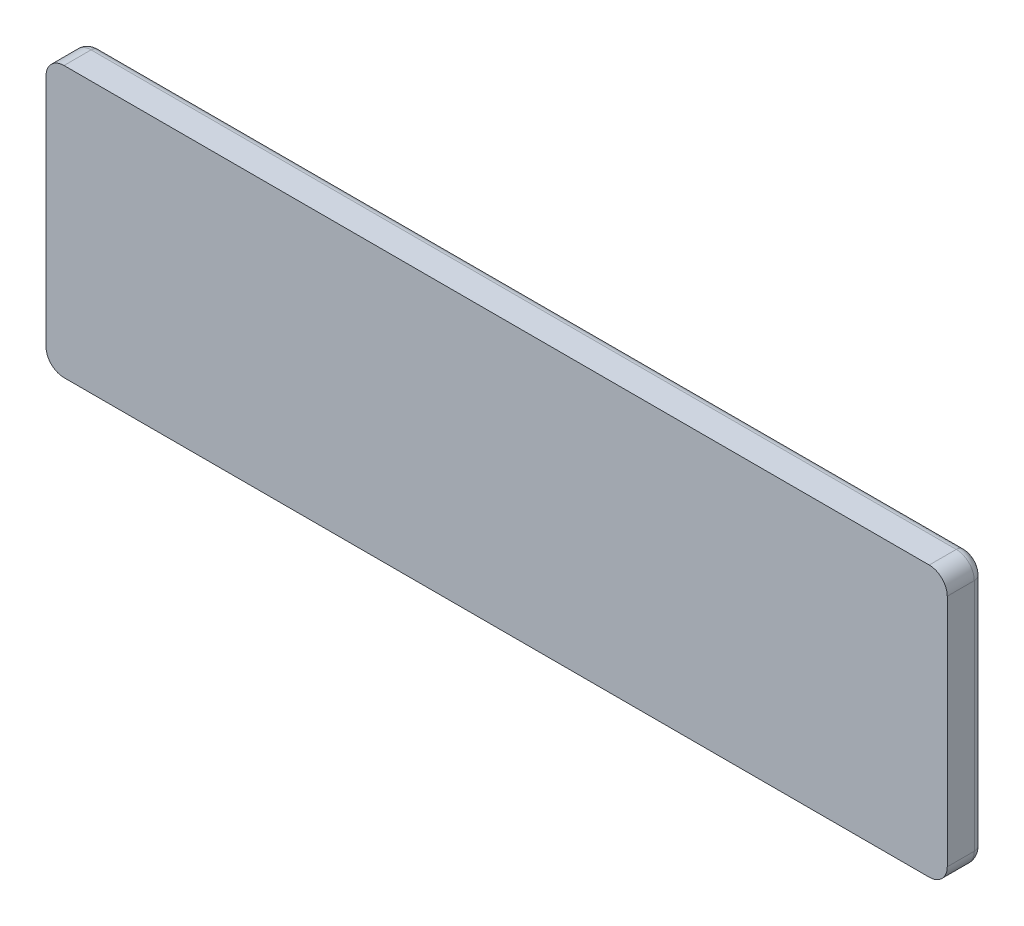
from build123d import *

# Parameters (mm, degrees)
BOSS_EXTRUDE1_DEPTH = 20
SKETCH2_W           = 15
SKETCH2_H           = 15
BOSS_EXTRUDE2_DEPTH = 4
SKETCH3_W           = 15
SKETCH3_H           = 15
BOSS_EXTRUDE3_DEPTH = 4
SKETCH4_W           = 15
SKETCH4_H           = 15
BOSS_EXTRUDE4_DEPTH = 4
SKETCH5_W           = 15
SKETCH5_H           = 15
BOSS_EXTRUDE5_DEPTH = 4
SKETCH6_W           = 15
SKETCH6_H           = 15
BOSS_EXTRUDE6_DEPTH = 4
SKETCH7_R           = 2
BOSS_EXTRUDE7_DEPTH = 1
FILLET2_R           = 10
FILLET3_R           = 5


with BuildPart() as part:
    # Sketch1 → Boss-Extrude1 (new body)
    with BuildSketch(Plane.XY):
        Polygon((0, 150), (-50, 150), (-50, 0), (0, 0), (450, 0), (450, 150), align=None)
    extrude(amount=BOSS_EXTRUDE1_DEPTH)

    # Sketch2 → Boss-Extrude2 (add)
    with BuildSketch(Plane(origin=(0, 0, 0), x_dir=(-1, 0, 0), z_dir=(0, 0, -1))):
        with Locations((-432.5, 132.5)):
            Rectangle(SKETCH2_W, SKETCH2_H)
    extrude(amount=BOSS_EXTRUDE2_DEPTH)

    # Sketch3 → Boss-Extrude3 (add)
    with BuildSketch(Plane(origin=(0, 0, 0), x_dir=(-1, 0, 0), z_dir=(0, 0, -1))):
        with Locations((-374.953657525, 132.5)):
            Rectangle(SKETCH3_W, SKETCH3_H)
        with Locations((-394.953657525, 132.5)):
            Rectangle(SKETCH3_W, SKETCH3_H)
        with Locations((-354.953657525, 132.5)):
            Rectangle(SKETCH3_W, SKETCH3_H)
        with Locations((-334.953657525, 132.5)):
            Rectangle(SKETCH3_W, SKETCH3_H)
        with Locations((-314.953657525, 132.5)):
            Rectangle(SKETCH3_W, SKETCH3_H)
        with Locations((-294.953657525, 132.5)):
            Rectangle(SKETCH3_W, SKETCH3_H)
        with Locations((-274.953657525, 132.5)):
            Rectangle(SKETCH3_W, SKETCH3_H)
        with Locations((-254.953657525, 132.5)):
            Rectangle(SKETCH3_W, SKETCH3_H)
        with Locations((-234.953657525, 132.5)):
            Rectangle(SKETCH3_W, SKETCH3_H)
        with Locations((-214.953657525, 132.5)):
            Rectangle(SKETCH3_W, SKETCH3_H)
        with Locations((-194.953657525, 132.5)):
            Rectangle(SKETCH3_W, SKETCH3_H)
        with Locations((-174.953657525, 132.5)):
            Rectangle(SKETCH3_W, SKETCH3_H)
        with Locations((-154.953657525, 132.5)):
            Rectangle(SKETCH3_W, SKETCH3_H)
        with Locations((-134.953657525, 132.5)):
            Rectangle(SKETCH3_W, SKETCH3_H)
        with Locations((-114.953657525, 132.5)):
            Rectangle(SKETCH3_W, SKETCH3_H)
    extrude(amount=BOSS_EXTRUDE3_DEPTH)

    # Sketch4 → Boss-Extrude4 (add)
    with BuildSketch(Plane(origin=(0, 0, 0), x_dir=(-1, 0, 0), z_dir=(0, 0, -1))):
        with Locations((-432.5, 107.5)):
            Rectangle(SKETCH4_W, SKETCH4_H)
        with Locations((-412.5, 107.5)):
            Rectangle(SKETCH4_W, SKETCH4_H)
        with Locations((-392.5, 107.5)):
            Rectangle(SKETCH4_W, SKETCH4_H)
        with Locations((-372.5, 107.5)):
            Rectangle(SKETCH4_W, SKETCH4_H)
        with Locations((-352.5, 107.5)):
            Rectangle(SKETCH4_W, SKETCH4_H)
        with Locations((-332.5, 107.5)):
            Rectangle(SKETCH4_W, SKETCH4_H)
        with Locations((-312.5, 107.5)):
            Rectangle(SKETCH4_W, SKETCH4_H)
        with Locations((-292.5, 107.5)):
            Rectangle(SKETCH4_W, SKETCH4_H)
        with Locations((-272.5, 107.5)):
            Rectangle(SKETCH4_W, SKETCH4_H)
        with Locations((-252.5, 107.5)):
            Rectangle(SKETCH4_W, SKETCH4_H)
        with Locations((-232.5, 107.5)):
            Rectangle(SKETCH4_W, SKETCH4_H)
        with Locations((-212.5, 107.5)):
            Rectangle(SKETCH4_W, SKETCH4_H)
        with Locations((-192.5, 107.5)):
            Rectangle(SKETCH4_W, SKETCH4_H)
        with Locations((-172.5, 107.5)):
            Rectangle(SKETCH4_W, SKETCH4_H)
        with Locations((-152.5, 107.5)):
            Rectangle(SKETCH4_W, SKETCH4_H)
        Polygon((-140, 115), (-140, 100), (-120, 100), (-105, 100), (-105, 115), (-120, 115), align=None)
        Polygon((-240, 27), (-225, 27), (-205, 27), (-185, 27), (-185, 12), (-200, 12), (-220, 12), (-240, 12), (-260, 12), (-280, 12), (-305, 12), (-325, 12), (-340, 12), (-340, 27), (-320, 27), (-300, 27), (-280, 27), (-260, 27), align=None)
        with Locations((-432.5, 85.5)):
            Rectangle(SKETCH4_W, SKETCH4_H)
        with Locations((-412.5, 85.5)):
            Rectangle(SKETCH4_W, SKETCH4_H)
        with Locations((-392.5, 85.5)):
            Rectangle(SKETCH4_W, SKETCH4_H)
        with Locations((-372.5, 85.5)):
            Rectangle(SKETCH4_W, SKETCH4_H)
        with Locations((-352.5, 85.5)):
            Rectangle(SKETCH4_W, SKETCH4_H)
        with Locations((-332.5, 85.5)):
            Rectangle(SKETCH4_W, SKETCH4_H)
        with Locations((-312.5, 85.5)):
            Rectangle(SKETCH4_W, SKETCH4_H)
        with Locations((-292.5, 85.5)):
            Rectangle(SKETCH4_W, SKETCH4_H)
        with Locations((-272.5, 85.5)):
            Rectangle(SKETCH4_W, SKETCH4_H)
        with Locations((-252.5, 85.5)):
            Rectangle(SKETCH4_W, SKETCH4_H)
        with Locations((-232.5, 85.5)):
            Rectangle(SKETCH4_W, SKETCH4_H)
        with Locations((-212.5, 85.5)):
            Rectangle(SKETCH4_W, SKETCH4_H)
        with Locations((-192.5, 85.5)):
            Rectangle(SKETCH4_W, SKETCH4_H)
        with Locations((-172.5, 85.5)):
            Rectangle(SKETCH4_W, SKETCH4_H)
        with Locations((-152.5, 85.5)):
            Rectangle(SKETCH4_W, SKETCH4_H)
        Polygon((-140, 93), (-140, 78), (-120, 78), (-120, 56), (-105, 56), (-105, 78), (-105, 93), (-120, 93), align=None)
        with Locations((-432.5, 63.5)):
            Rectangle(SKETCH4_W, SKETCH4_H)
        with Locations((-412.5, 63.5)):
            Rectangle(SKETCH4_W, SKETCH4_H)
        with Locations((-392.5, 63.5)):
            Rectangle(SKETCH4_W, SKETCH4_H)
        with Locations((-372.5, 63.5)):
            Rectangle(SKETCH4_W, SKETCH4_H)
        with Locations((-352.5, 63.5)):
            Rectangle(SKETCH4_W, SKETCH4_H)
        with Locations((-332.5, 63.5)):
            Rectangle(SKETCH4_W, SKETCH4_H)
        with Locations((-312.5, 63.5)):
            Rectangle(SKETCH4_W, SKETCH4_H)
        with Locations((-292.5, 63.5)):
            Rectangle(SKETCH4_W, SKETCH4_H)
        with Locations((-272.5, 63.5)):
            Rectangle(SKETCH4_W, SKETCH4_H)
        with Locations((-252.5, 63.5)):
            Rectangle(SKETCH4_W, SKETCH4_H)
        with Locations((-232.5, 63.5)):
            Rectangle(SKETCH4_W, SKETCH4_H)
        with Locations((-212.5, 63.5)):
            Rectangle(SKETCH4_W, SKETCH4_H)
        with Locations((-192.5, 63.5)):
            Rectangle(SKETCH4_W, SKETCH4_H)
        with Locations((-172.5, 63.5)):
            Rectangle(SKETCH4_W, SKETCH4_H)
        with Locations((-152.5, 63.5)):
            Rectangle(SKETCH4_W, SKETCH4_H)
        with Locations((-132.5, 63.5)):
            Rectangle(SKETCH4_W, SKETCH4_H)
        with Locations((-432.5, 41.5)):
            Rectangle(SKETCH4_W, SKETCH4_H)
        with Locations((-412.5, 41.5)):
            Rectangle(SKETCH4_W, SKETCH4_H)
        with Locations((-392.5, 41.5)):
            Rectangle(SKETCH4_W, SKETCH4_H)
        with Locations((-372.5, 41.5)):
            Rectangle(SKETCH4_W, SKETCH4_H)
        with Locations((-352.5, 41.5)):
            Rectangle(SKETCH4_W, SKETCH4_H)
        with Locations((-332.5, 41.5)):
            Rectangle(SKETCH4_W, SKETCH4_H)
        with Locations((-312.5, 41.5)):
            Rectangle(SKETCH4_W, SKETCH4_H)
        with Locations((-292.5, 41.5)):
            Rectangle(SKETCH4_W, SKETCH4_H)
        with Locations((-272.5, 41.5)):
            Rectangle(SKETCH4_W, SKETCH4_H)
        with Locations((-252.5, 41.5)):
            Rectangle(SKETCH4_W, SKETCH4_H)
        with Locations((-232.5, 41.5)):
            Rectangle(SKETCH4_W, SKETCH4_H)
        with Locations((-212.5, 41.5)):
            Rectangle(SKETCH4_W, SKETCH4_H)
        with Locations((-192.5, 41.5)):
            Rectangle(SKETCH4_W, SKETCH4_H)
        with Locations((-172.5, 41.5)):
            Rectangle(SKETCH4_W, SKETCH4_H)
        with Locations((-152.5, 41.5)):
            Rectangle(SKETCH4_W, SKETCH4_H)
        Polygon((-140, 49), (-140, 34), (-125, 34), (-105, 34), (-105, 49), (-125, 49), align=None)
        with Locations((-432.5, 19.5)):
            Rectangle(SKETCH4_W, SKETCH4_H)
        with Locations((-412.5, 19.5)):
            Rectangle(SKETCH4_W, SKETCH4_H)
        with Locations((-392.5, 19.5)):
            Rectangle(SKETCH4_W, SKETCH4_H)
        with Locations((-372.5, 19.5)):
            Rectangle(SKETCH4_W, SKETCH4_H)
        with Locations((-352.5, 19.5)):
            Rectangle(SKETCH4_W, SKETCH4_H)
        with Locations((-172.5, 19.5)):
            Rectangle(SKETCH4_W, SKETCH4_H)
        with Locations((-152.5, 19.5)):
            Rectangle(SKETCH4_W, SKETCH4_H)
        with Locations((-132.5, 19.5)):
            Rectangle(SKETCH4_W, SKETCH4_H)
    extrude(amount=BOSS_EXTRUDE4_DEPTH)

    # Sketch5 → Boss-Extrude5 (add)
    with BuildSketch(Plane(origin=(0, 0, 0), x_dir=(-1, 0, 0), z_dir=(0, 0, -1))):
        with Locations((-89.953657525, 132.5)):
            Rectangle(SKETCH5_W, SKETCH5_H)
        with Locations((-69.953657525, 132.5)):
            Rectangle(SKETCH5_W, SKETCH5_H)
        with Locations((-49.953657525, 132.5)):
            Rectangle(SKETCH5_W, SKETCH5_H)
        with Locations((-69.953657525, 107.5)):
            Rectangle(SKETCH5_W, SKETCH5_H)
        with Locations((-89.953657525, 107.5)):
            Rectangle(SKETCH5_W, SKETCH5_H)
        with Locations((-49.953657525, 107.5)):
            Rectangle(SKETCH5_W, SKETCH5_H)
        with Locations((-89.953657525, 85.5)):
            Rectangle(SKETCH5_W, SKETCH5_H)
        with Locations((-69.953657525, 85.5)):
            Rectangle(SKETCH5_W, SKETCH5_H)
        with Locations((-49.953657525, 85.5)):
            Rectangle(SKETCH5_W, SKETCH5_H)
        with Locations((-69.953657525, 41.5)):
            Rectangle(SKETCH5_W, SKETCH5_H)
        with Locations((-89.953657525, 19.5)):
            Rectangle(SKETCH5_W, SKETCH5_H)
        with Locations((-69.953657525, 19.5)):
            Rectangle(SKETCH5_W, SKETCH5_H)
        with Locations((-49.953657525, 19.5)):
            Rectangle(SKETCH5_W, SKETCH5_H)
    extrude(amount=BOSS_EXTRUDE5_DEPTH)

    # Sketch6 → Boss-Extrude6 (add)
    with BuildSketch(Plane(origin=(0, 0, 0), x_dir=(-1, 0, 0), z_dir=(0, 0, -1))):
        with Locations((-2.953657525, 107.5)):
            Rectangle(SKETCH6_W, SKETCH6_H)
        with Locations((-22.953657525, 107.5)):
            Rectangle(SKETCH6_W, SKETCH6_H)
        with Locations((17.046342475, 107.5)):
            Rectangle(SKETCH6_W, SKETCH6_H)
        with Locations((37.046342475, 107.5)):
            Rectangle(SKETCH6_W, SKETCH6_H)
        with Locations((-22.953657525, 85.5)):
            Rectangle(SKETCH6_W, SKETCH6_H)
        with Locations((-2.953657525, 85.5)):
            Rectangle(SKETCH6_W, SKETCH6_H)
        with Locations((17.046342475, 85.5)):
            Rectangle(SKETCH6_W, SKETCH6_H)
        Polygon((29.546342475, 93), (44.546342475, 93), (44.546342475, 78), (44.546342475, 56), (29.546342475, 56), (29.546342475, 78), align=None)
        with Locations((-22.953657525, 63.5)):
            Rectangle(SKETCH6_W, SKETCH6_H)
        with Locations((-2.953657525, 63.5)):
            Rectangle(SKETCH6_W, SKETCH6_H)
        with Locations((17.046342475, 63.5)):
            Rectangle(SKETCH6_W, SKETCH6_H)
        with Locations((-22.953657525, 41.5)):
            Rectangle(SKETCH6_W, SKETCH6_H)
        with Locations((-2.953657525, 41.5)):
            Rectangle(SKETCH6_W, SKETCH6_H)
        with Locations((17.046342475, 41.5)):
            Rectangle(SKETCH6_W, SKETCH6_H)
        Polygon((29.546342475, 49), (44.546342475, 49), (44.546342475, 27), (44.546342475, 12), (29.546342475, 12), (29.546342475, 27), align=None)
        Polygon((-30.453657525, 27), (-15.453657525, 27), (4.546342475, 27), (4.546342475, 12), (-10.453657525, 12), (-30.453657525, 12), align=None)
        with Locations((17.046342475, 19.5)):
            Rectangle(SKETCH6_W, SKETCH6_H)
    extrude(amount=BOSS_EXTRUDE6_DEPTH)

    # Sketch7 → Boss-Extrude7 (add)
    with BuildSketch(Plane(origin=(0, 0, 0), x_dir=(-1, 0, 0), z_dir=(0, 0, -1))):
        with Locations(Location((-17.453657525, 132.5, 0), (0, 0, 180))):
            Circle(SKETCH7_R)
        with Locations(Location((7.546342475, 132.5, 0), (0, 0, 180))):
            Circle(SKETCH7_R)
        with Locations(Location((32.546342475, 132.5, 0), (0, 0, 180))):
            Circle(SKETCH7_R)
    extrude(amount=BOSS_EXTRUDE7_DEPTH)

    # Fillet2
    fillet2_edges = [part.edges().sort_by_distance(p)[0] for p in [
        (-50, 0, 10),
        (-50, 150, 10),
        (450, 150, 10),
        (450, 0, 10),
    ]]
    fillet(fillet2_edges, radius=FILLET2_R)

    # Fillet3
    fillet3_edges = [part.edges().sort_by_distance(p)[0] for p in [
        (-50, 75, 0),
        (200, 0, 0),
        (200, 150, 0),
        (450, 75, 0),
        (447.071067812, 2.928932188, 0),
        (447.071067812, 147.071067812, 0),
        (-47.071067812, 2.928932188, 0),
        (-47.071067812, 147.071067812, 0),
    ]]
    fillet(fillet3_edges, radius=FILLET3_R)


solid = part.part
